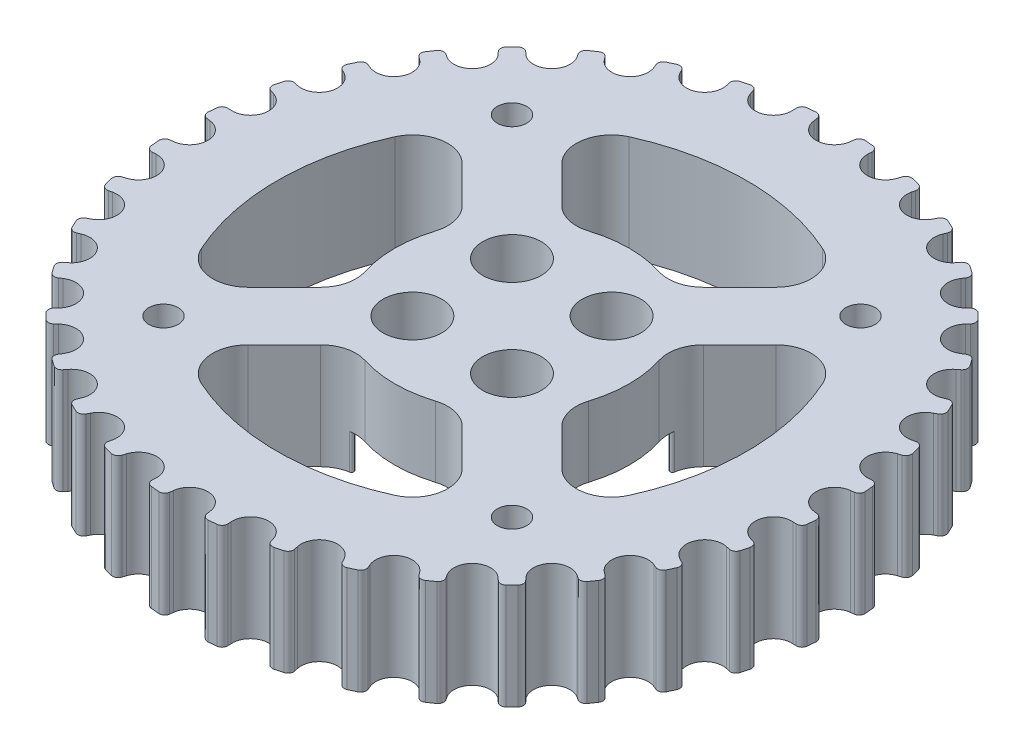
SolidWorks part; units mm, degrees
material "6061 合金"
ref_plane "前视基准面" through (0, 0, 0) normal (0, 0, 1) x (1, 0, 0)
ref_plane "上视基准面" through (0, 0, 0) normal (0, 1, 0) x (1, 0, 0)
ref_plane "右视基准面" through (0, 0, 0) normal (1, 0, 0) x (0, 0, -1)
sketch "草图1" plane through (0, 0, 0) normal (0, 0, 1) x (1, 0, 0)
  line L0 (24, 0) -> (28.08, 0)
  line L1 (28.08, 0) -> (28.08, 9)
  line L2 (28.08, 9) -> (30.1479, 9)
  line L3 (30.1479, 9) -> (30.1479, 11.5)
  line L4 (30.1479, 11.5) -> (22.5, 11.5)
  line L5 (22.5, 11.5) -> (22.5, 4)
  line L6 (22.5, 4) -> (18, 4)
  line L7 (9, 3) -> (9, -2)
  line L8 (21, 2) -> (24, 2)
  line L9 (24, 2) -> (24, 0)
  line L10 (0, 0) -> (24, 0) construction
  line L11 (0, 0) -> (0, 11.5) construction
  line L12 (9, 3) -> (18, 3)
  line L13 (18, 3) -> (18, 4)
  line L14 (21, 2) -> (21, -5)
  line L15 (21, -5) -> (20, -5)
  line L16 (20, -5) -> (20, -6)
  line L17 (20, -6) -> (18.5, -6)
  line L18 (9, -2) -> (18.5, -2)
  line L19 (18.5, -2) -> (18.5, -6)
  dimension "D1" = 22.5
  dimension "D2" = 24
  dimension "D3" = 2
  dimension "D4" = 9
  dimension "D5" = 2.5
  dimension "D6" = 9
  dimension "D7" = 7.5
  dimension "D8" = 28.08
  dimension "D9" = 30.1479
  dimension "D10" = 18
  dimension "D11" = 1
  dimension "D12" = 21
  dimension "D13" = 20
  dimension "D14" = 1
  dimension "D15" = 5
  dimension "D16" = 4
  dimension "D17" = 18.5
revolve "旋转1" add sketch "草图1" angle 360 about L11
sketch "草图2" plane through (0, 9, 0) normal (0, -1, 0) x (1, 0, 0)
  line L0 (0, 0) -> (0, 28.08) construction
  line L1 (-1.5842, 27.5815) -> (-1.5484, 27.2899)
  line L2 (1.5842, 27.5815) -> (1.5484, 27.2899)
  arc A2 (-1.5484, 27.2899) -> (1.5484, 27.2899) centre (0, 27.48) ccw
  arc A3 (1.5842, 27.5815) -> (2.0964, 28.0016) centre (2.0606, 27.523) cw
  arc A4 (-1.5842, 27.5815) -> (-2.0964, 28.0016) centre (-2.0606, 27.523) ccw
  circle A5 centre (0, 0) radius 28.08 construction
  arc A6 (2.0964, 28.0016) -> (-2.0964, 28.0016) centre (0, 0) ccw
  point P17 (0, 25.92)
  dimension "D1" = 0.48
  dimension "D2" = 1.56
  dimension "D3" = 14
  dimension "D4" = 2.16
extrude "切除-拉伸1" cut sketch "草图2" along normal through all
pattern_circular "阵列(圆周)1" count 36 over 360 about axis through (0, 0, 0) along (0, 1, 0) of "切除-拉伸1"
sketch "草图3" plane through (0, 11.5, 0) normal (0, 1, 0) x (1, 0, 0)
  circle A0 centre (0, 0) radius 41.8465
extrude "切除-拉伸2" cut sketch "草图3" against normal up to surface (2.5 mm away)
sketch "草图4" plane through (0, 9, 0) normal (0, 1, 0) x (1, 0, 0)
  circle A0 centre (0, 0) radius 25
  dimension "D1" = 50
extrude "凸台-拉伸1" add sketch "草图4" against normal up to surface (9 mm away) up to face at (0, 0, -24)
sketch "草图5" plane through (0, -6, 0) normal (0, -1, 0) x (1, 0, 0)
  circle A0 centre (0, 0) radius 29.3651
extrude "切除-拉伸3" cut sketch "草图5" against normal up to surface (6 mm away)
sketch "草图6" plane through (0, 9, 0) normal (0, 1, 0) x (1, 0, 0)
  line L0 (-6.0334, 10.2761) -> (-9.1259, 13.3685)
  line L1 (-4.2426, -4.2426) -> (4.2426, -4.2426) construction
  line L2 (-4.2426, -4.2426) -> (-4.2426, 4.2426) construction
  line L3 (-4.2426, 4.2426) -> (4.2426, 4.2426) construction
  line L4 (4.2426, -4.2426) -> (4.2426, 4.2426) construction
  line L5 (-4.2426, -4.2426) -> (4.2426, 4.2426) construction
  line L6 (-4.2426, 4.2426) -> (4.2426, -4.2426) construction
  line L7 (-13.3685, 9.1259) -> (-10.2761, 6.0334)
  line L8 (10.2761, 6.0334) -> (13.3685, 9.1259)
  line L9 (9.1259, 13.3685) -> (6.0334, 10.2761)
  line L10 (6.0334, -10.2761) -> (9.1259, -13.3685)
  line L11 (13.3685, -9.1259) -> (10.2761, -6.0334)
  line L12 (-10.2761, -6.0334) -> (-13.3685, -9.1259)
  line L13 (-9.1259, -13.3685) -> (-6.0334, -10.2761)
  arc A0 (-18.2234, 8.2407) -> (-18.2234, -8.2407) centre (0, 0) ccw
  circle A1 centre (-4.2426, 4.2426) radius 2.5
  circle A2 centre (4.2426, 4.2426) radius 2.5
  circle A3 centre (-4.2426, -4.2426) radius 2.5
  circle A4 centre (4.2426, -4.2426) radius 2.5
  arc A5 (-3.0093, -9.5365) -> (3.0093, -9.5365) centre (0, 0) ccw
  arc A6 (8.2407, 18.2234) -> (-8.2407, 18.2234) centre (0, 0) ccw
  arc A7 (-8.2407, -18.2234) -> (8.2407, -18.2234) centre (0, 0) ccw
  arc A8 (9.5365, -3.0093) -> (9.5365, 3.0093) centre (0, 0) ccw
  arc A9 (3.0093, 9.5365) -> (-3.0093, 9.5365) centre (0, 0) ccw
  arc A10 (-9.5365, 3.0093) -> (-9.5365, -3.0093) centre (0, 0) ccw
  arc A11 (18.2234, -8.2407) -> (18.2234, 8.2407) centre (0, 0) ccw
  arc A12 (10.2761, -6.0334) -> (9.5365, -3.0093) centre (12.3974, -3.9121) cw
  arc A13 (10.2761, 6.0334) -> (9.5365, 3.0093) centre (12.3974, 3.9121) ccw
  arc A14 (13.3685, 9.1259) -> (18.2234, 8.2407) centre (15.4899, 7.0046) cw
  arc A15 (13.3685, -9.1259) -> (18.2234, -8.2407) centre (15.4899, -7.0046) ccw
  arc A16 (9.1259, -13.3685) -> (8.2407, -18.2234) centre (7.0046, -15.4899) cw
  arc A17 (-9.1259, -13.3685) -> (-8.2407, -18.2234) centre (-7.0046, -15.4899) ccw
  arc A18 (6.0334, -10.2761) -> (3.0093, -9.5365) centre (3.9121, -12.3974) ccw
  arc A19 (-6.0334, -10.2761) -> (-3.0093, -9.5365) centre (-3.9121, -12.3974) cw
  arc A20 (-9.1259, 13.3685) -> (-8.2407, 18.2234) centre (-7.0046, 15.4899) cw
  arc A21 (9.1259, 13.3685) -> (8.2407, 18.2234) centre (7.0046, 15.4899) ccw
  arc A22 (6.0334, 10.2761) -> (3.0093, 9.5365) centre (3.9121, 12.3974) cw
  arc A23 (-6.0334, 10.2761) -> (-3.0093, 9.5365) centre (-3.9121, 12.3974) ccw
  arc A24 (-10.2761, 6.0334) -> (-9.5365, 3.0093) centre (-12.3974, 3.9121) cw
  arc A25 (-10.2761, -6.0334) -> (-9.5365, -3.0093) centre (-12.3974, -3.9121) ccw
  arc A26 (-13.3685, -9.1259) -> (-18.2234, -8.2407) centre (-15.4899, -7.0046) cw
  arc A27 (-13.3685, 9.1259) -> (-18.2234, 8.2407) centre (-15.4899, 7.0046) ccw
  circle A28 centre (-14.8492, 14.8492) radius 1.25
  circle A29 centre (0, 0) radius 21 construction
  circle A30 centre (14.8492, 14.8492) radius 1.25
  circle A31 centre (14.8492, -14.8492) radius 1.25
  circle A32 centre (-14.8492, -14.8492) radius 1.25
  point P31 (0, 0)
  point P52 (-4.624, 8.8667)
  point P55 (-8.8667, 4.624)
  point P73 (0, 0)
  dimension "D1" = 40
  dimension "D2" = 5
  dimension "D4" = 20
  dimension "D7" = 3
  dimension "D8" = 42
  dimension "D9" = 2.5
  dimension "D3" = 6
  dimension "D5" = 3
  dimension "D6" = 4
  dimension "D10" = 4
extrude "切除-拉伸4" cut sketch "草图6" against normal blind 10
sketch "草图8" plane through (0, 0, 0) normal (0, -1, 0) x (1, 0, 0)
  circle A0 centre (0, 0) radius 10.05
  dimension "D1" = 20.1
extrude "切除-拉伸6" cut sketch "草图8" against normal blind 3
chamfer "倒角1" [suppressed] distance 1 angle 45
fillet "圆角1" radius 0.2 8 edges at (3.4781, 1.5, 9.4289) (9.4289, 1.5, 3.4781) (9.4289, 1.5, -3.4781) (3.4781, 1.5, -9.4289) (-3.4781, 1.5, -9.4289) (-9.4289, 1.5, -3.4781) (-9.4289, 1.5, 3.4781) (-3.4781, 1.5, 9.4289)
